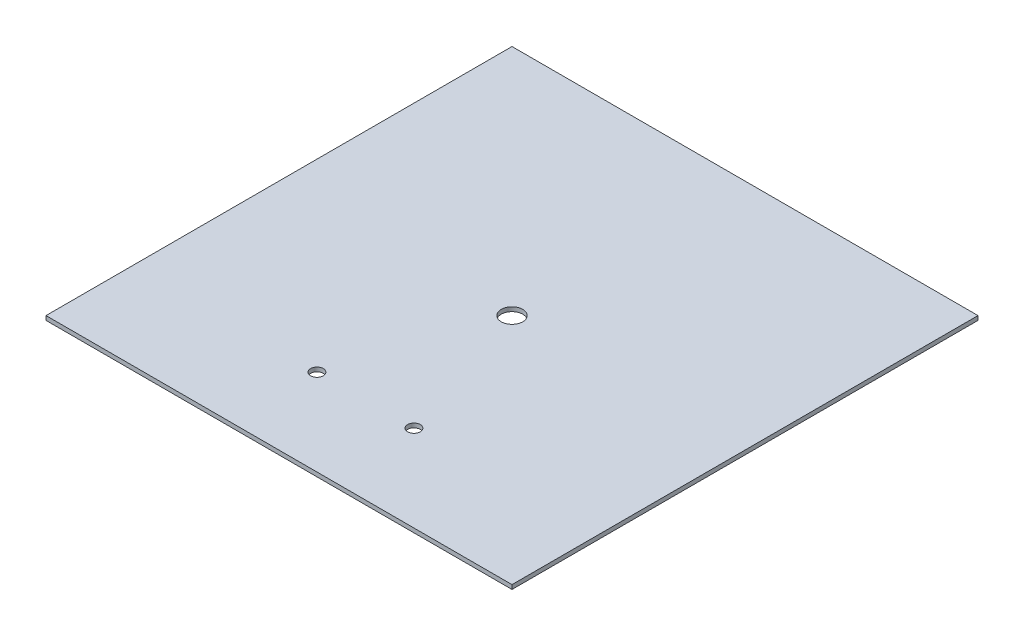
SolidWorks part; units mm, degrees
ref_plane "Front Plane" through (0, 0, 0) normal (0, 0, 1) x (1, 0, 0)
ref_plane "Top Plane" through (0, 0, 0) normal (0, 1, 0) x (1, 0, 0)
ref_plane "Right Plane" through (0, 0, 0) normal (1, 0, 0) x (0, 0, -1)
sketch "Sketch1" plane through (0, 0, 0) normal (0, 1, 0) x (1, 0, 0)
  line L0 (0, 55.25) -> (0, -55.25) construction
  line L1 (-55.25, -55.25) -> (55.25, -55.25)
  line L2 (-55.25, -55.25) -> (-55.25, 55.25)
  line L3 (-55.25, 55.25) -> (55.25, 55.25)
  line L4 (55.25, -55.25) -> (55.25, 55.25)
  line L5 (-55.25, -55.25) -> (55.25, 55.25) construction
  line L6 (-55.25, 55.25) -> (55.25, -55.25) construction
  circle A0 centre (0, 0) radius 2.55
  circle A1 centre (-11.5, -34.75) radius 1.5
  circle A2 centre (11.5, -34.75) radius 1.5
  point P0 (0, 0)
  dimension "D2" = 5.1
  dimension "D3" = 23
  dimension "D5" = 3
  dimension "D1" = 110.5
  dimension "D4" = 20.5
extrude "Boss-Extrude1" add sketch "Sketch1" along normal blind 1
